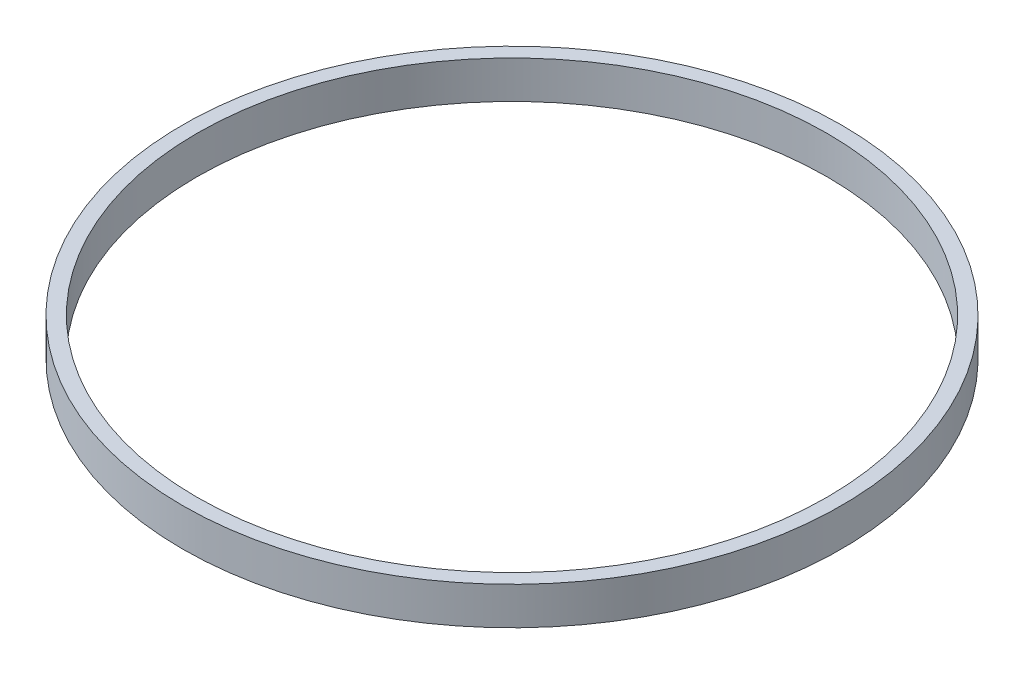
SolidWorks part; units mm, degrees
ref_plane "Front Plane" through (0, 0, 0) normal (0, 0, 1) x (1, 0, 0)
ref_plane "Top Plane" through (0, 0, 0) normal (0, 1, 0) x (1, 0, 0)
ref_plane "Right Plane" through (0, 0, 0) normal (1, 0, 0) x (0, 0, -1)
sketch "Sketch1" plane through (0, 0, 0) normal (0, 1, 0) x (1, 0, 0)
  circle A0 centre (0, 0) radius 26.25
  circle A1 centre (0, 0) radius 25.1
  dimension "D1" = 50.2
  dimension "D2" = 52.5
extrude "Boss-Extrude1" add sketch "Sketch1" along normal blind 3
